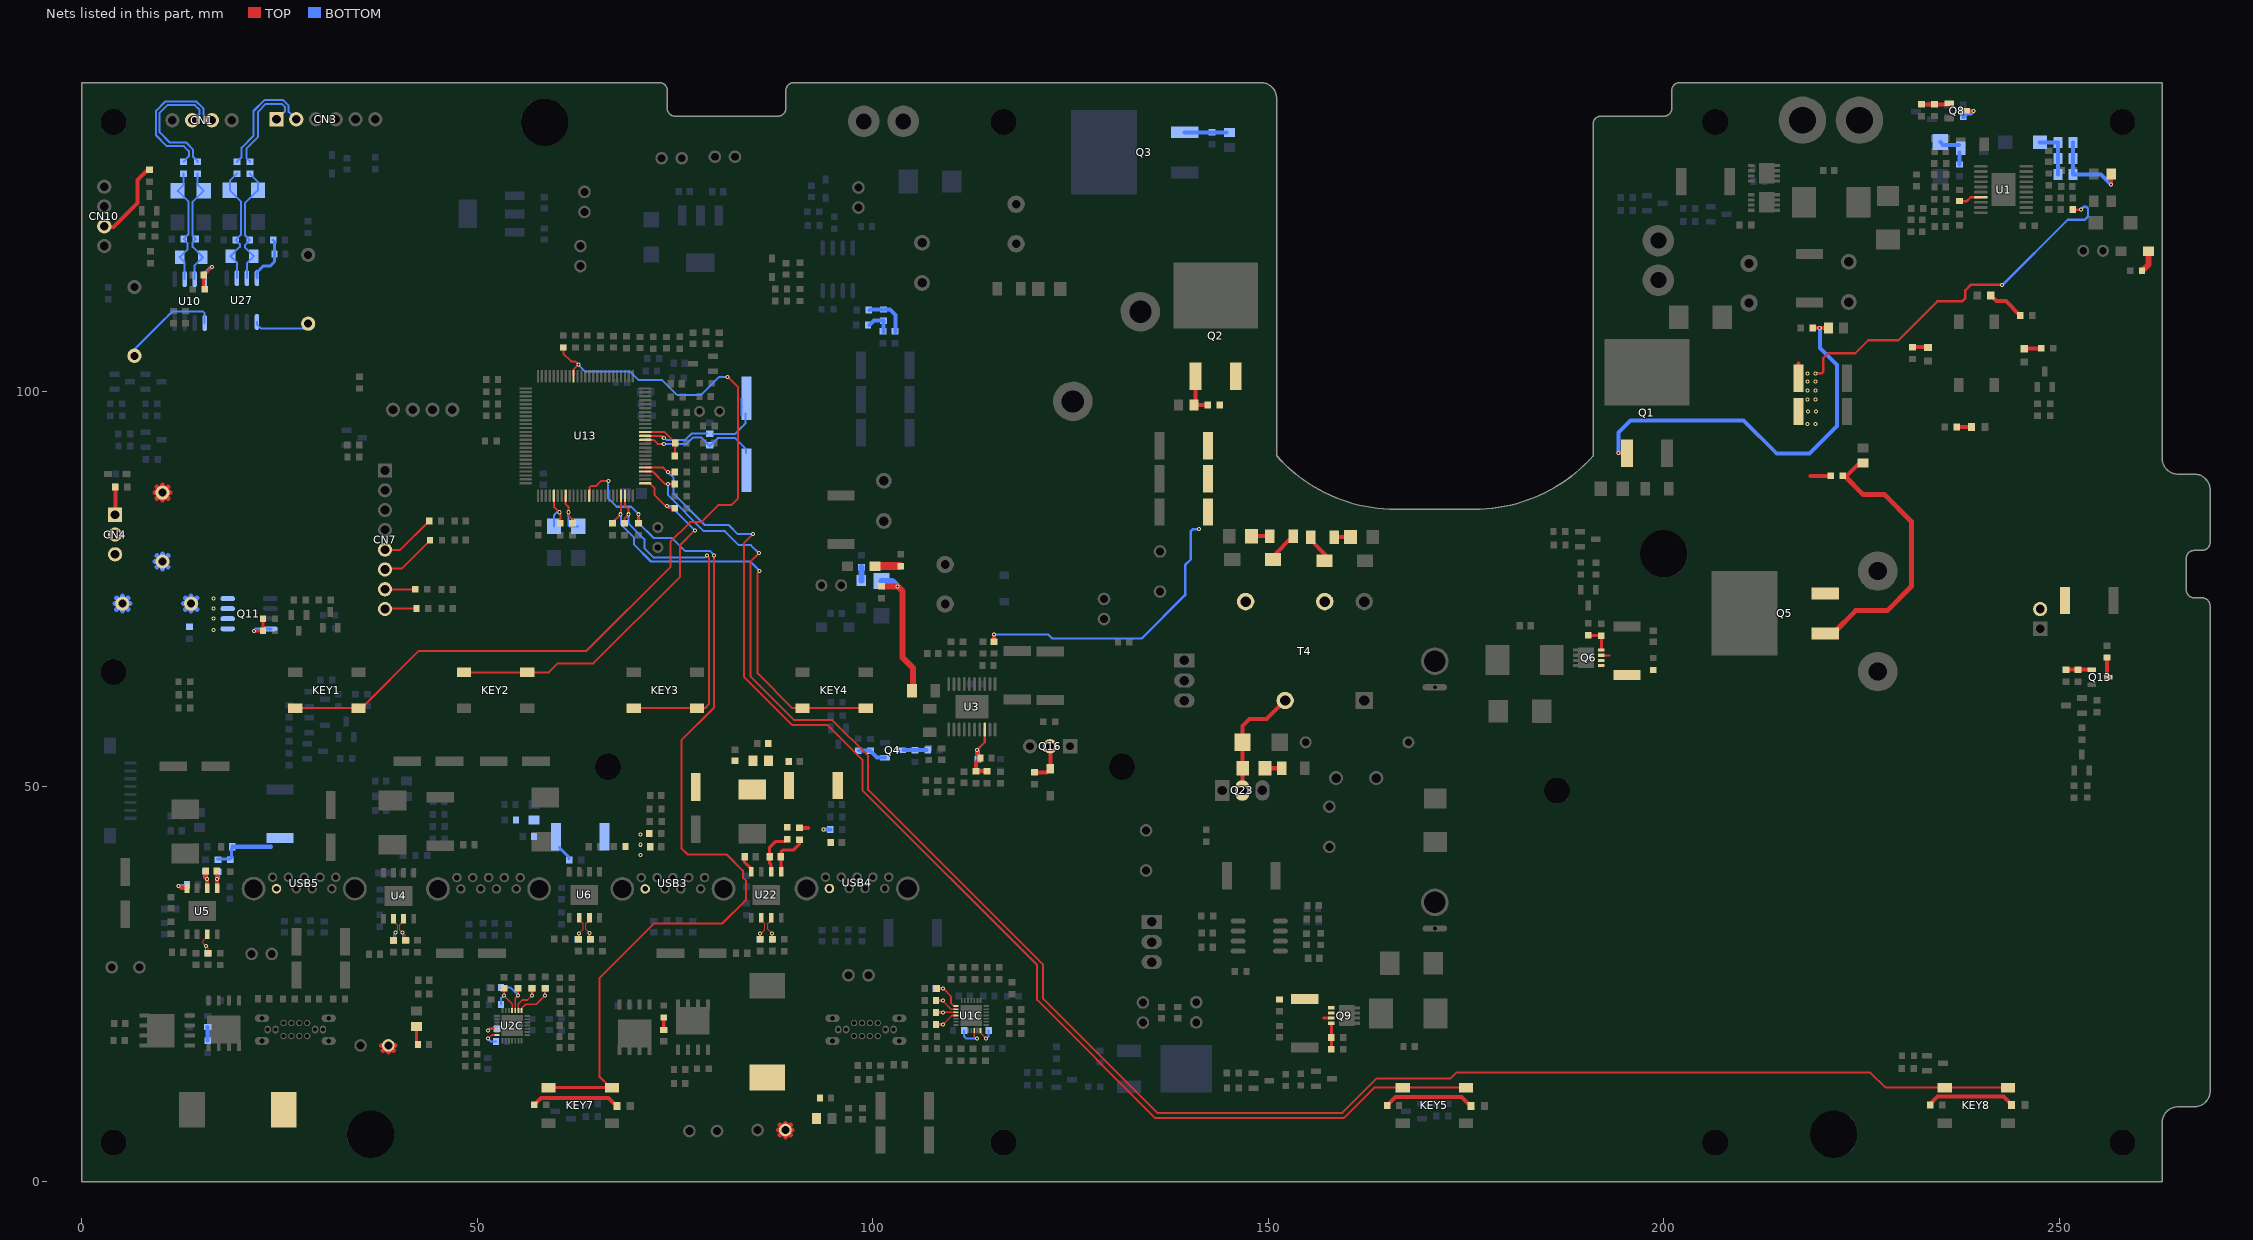
[diagram p0: the nets of this part, all layers, seen from the top]
# Altium PCB MISC84402.PcbDoc (part 7 of 12)
Units mm, origin at the board's own origin, x right, y up, seen from the top; angles counter-clockwise.
Board outline 269.06 x 139 mm, 4 copper layers (TOP, GND02, PWR03, BOTTOM), stack 0.732 mm thick; 694 components, 428 nets, 1859 pads, 1384 vias.

## Via types
v1: diameter 0.508, hole 0.254, TOP to BOTTOM, tented both sides, 1015 vias
v2: diameter 0.508, hole 0.254, TOP to BOTTOM, 243 vias
v3: diameter 0.508, hole 0.305, TOP to BOTTOM, 60 vias
v4: diameter 0.61, hole 0.305, TOP to BOTTOM, 55 vias
v5: diameter 0.61, hole 0.305, TOP to BOTTOM, tented both sides, 8 vias
v6: diameter 0.762, hole 0.381, TOP to BOTTOM, 2 vias
v7: diameter 0.762, hole 0.381, TOP to BOTTOM, tented both sides, 1 vias

## Nets (pads, with @x,y where several pads share a name; then routed paths per layer and width w, separated by ;. In a path a pad name is that pad's centre, name@x,y a point inside that pad or via, vN(x,y) a via of type N, cw(c..) or ccw(c..) an arc to the next point about the centre after c; other vN are vias at no path point) (continued)
NETC107_1: C107.1 C113.2 L6.2 L13.1 | length 7.1
  TOP w0.635: 88.075,6.569 C107.1@88.926,6.569 ; 88.273,5.916 C107.1@88.926,6.569 ; 88.273,7.221 C107.1@88.926,6.569 ; 88.926,5.717 C107.1@88.926,6.569 ; 88.926,7.42 C107.1@88.926,6.569 ; 89.579,5.916 C107.1@88.926,6.569 ; 89.579,7.221 C107.1@88.926,6.569 ; 89.777,6.569 C107.1@88.926,6.569
NETC108_1: C108.1 R166.2 U1C.3 | length 3.4
  TOP w0.203: C108.1@108.179,21.463 108.195,21.447 U1C.3@110.513,21.447
  TOP w0.254: C108.1@107.978,21.428 C108.1@108.179,21.428
  BOTTOM w0.254: R166.2@107.978,21.428 v1(108.865,21.428)
NETC109_1: C109.1 R204.2 U2C.3 | length 5.5
  TOP w0.203: U2C.3@54.782,21.684 54.782,23.225 v1(55.144,23.587)
  TOP w0.254: v1(55.144,23.587) C109.1@55.144,24.476
  BOTTOM w0.254: R204.2@52.976,24.603 54.128,24.603 v1(55.144,23.587)
NETC110_1: C110.1 R160.2 U1C.1 | length 4.8
  TOP w0.203: R160.2@108.28,24.486 108.89,24.486 109.88,23.495 109.88,22.581 110.214,22.247 U1C.1@110.513,22.247
  TOP w0.254: R160.2@108.083,24.476 R160.2@108.28,24.476
  BOTTOM w0.254: C110.1@107.976,24.476 v1(108.867,24.476)
NETC111_1: C111.1 R205.2 U2C.2 | length 4.8
  TOP w0.203: U2C.2@55.182,21.684 55.182,22.543 55.651,23.012 56.337,23.012 56.972,23.647 C111.1@56.972,24.333
  TOP w0.254: C111.1@56.922,24.333 C111.1@56.922,24.476
  BOTTOM w0.254: v1(56.922,23.587) R205.2@56.922,24.476
NETC115_1: C115.1 C129.2 L7.2 L12.1 | length 6.8
  TOP w0.381: L12.1@42.291,19.685 42.291,17.588 C129.2@42.48,17.399
  TOP w0.635: 37.882,17.265 C115.1@38.733,17.265 ; 38.08,16.612 C115.1@38.733,17.265 ; 38.733,16.413 C115.1@38.733,17.265 ; 39.386,16.612 C115.1@38.733,17.265 ; 39.584,17.265 C115.1@38.733,17.265
NetC117_2: C117.2 C142.2 L11.2 R82.2 R340.1 | length 1.9
  BOTTOM w0.381: R82.2@60.376,42.266 61.578,41.063 R340.1@61.578,40.853
NETC118_1: C118.1 R229.1 U10.8 | length 5.3
  TOP w0.381: R229.1@15.52,112.868 15.395,112.992 C118.1@15.395,114.646 v1(16.431,115.681)
  BOTTOM w0.381: U10.8@15.52,114.138 15.52,114.9 16.301,115.681 v1(16.431,115.681)
NETC119_2: C119.2 R174.1 | length 1.6
  TOP w0.381: C119.2@73.559,19.207 R174.1@73.559,20.801
NETC120_2: C120.2 U1C.14 | length 2.5
  TOP w0.203: U1C.14@113.621,19.139 113.621,18.84 v1@114.3,18.161
  TOP w0.254: v1@114.295,18.156 v1(114.326,18.126)
  BOTTOM w0.254: v1(114.326,18.126) 114.645,18.444 C120.2@114.645,19.142
NETC121_2: C121.2 U2C.12 | length 2.5
  TOP w0.203: v1@51.333,19.101 51.609,19.377 U2C.12@52.474,19.377
  BOTTOM w0.254: v1(51.334,19.142) 51.569,19.377 C121.2@52.474,19.377
NetC123_2: C123.2 C150.2 L14.2 R83.2 R339.1
NETC124_1: C124.1 R231.1 U27.8 | length 6.3
  BOTTOM w0.381: U27.8@22.124,114.265 22.124,115.027 22.886,115.789 23.775,115.789 24.345,116.359 C124.1@24.345,117.313 24.345,118.91 R231.1@24.165,119.091
NetC130_2: C130.2 R7.2 R8.1 R14.1 U3.8 | length 8.7
  TOP w0.305: v1(113.157,54.61) 114.147,55.6 U3.8@114.147,57.198
  TOP w0.508: v1(113.157,54.61) 113.157,54.037 C130.2@113.6,53.594 113.03,53.024 R14.1@113.03,51.934 R8.1@114.427,51.934
  BOTTOM w0.508: v1(113.157,54.61) 113.284,54.483 R7.2@113.284,53.467
NETC132_1: C132.1 R203.2 U2C.1 | length 5.7
  TOP w0.203: U2C.1@55.582,21.684 55.582,21.952 56.109,22.479 57.455,22.479 58.572,23.597 R203.2@58.572,24.359
  TOP w0.254: R203.2@58.573,24.359 R203.2@58.573,24.476
  BOTTOM w0.254: v1(58.573,23.587) C132.1@58.573,24.476
NETC134_1: C134.1 R208.2 U2C.4 | length 4.5
  TOP w0.203: C134.1@53.391,24.409 53.391,23.562 53.391,23.52 54.382,22.529 U2C.4@54.382,21.684
  TOP w0.254: C134.1@53.366,24.409 C134.1@53.366,24.476
  BOTTOM w0.254: R208.2@52.976,22.444 52.976,23.197 v1(53.366,23.587)
NETC135_1: C135.1 R164.2 U1C.2 | length 3.9
  TOP w0.203: C135.1@108.026,22.936 108.788,22.936 109.878,21.847 U1C.2@110.513,21.847
  TOP w0.254: C135.1@107.978,22.952 C135.1@108.026,22.952
  BOTTOM w0.254: R164.2@107.978,22.952 v1(108.865,22.952)
NETC136_2: C136.2 U2C.14 | length 2.5
  TOP w0.203: v1@51.384,18.161 51.8,18.577 U2C.14@52.474,18.577
  TOP w0.254: v1(51.334,18.126) v1@51.377,18.168
  BOTTOM w0.254: v1(51.334,18.126) 51.715,17.745 C136.2@52.35,17.745
NETC139_2: C139.2 R226.1 | length 1.7
  BOTTOM w0.508: R226.1@15.901,17.863 C139.2@15.901,19.585
NETC143_1: C143.1 R344.2 U5.1 | length 3.3
  TOP w0.508: C143.1@17.046,39.335 v1(17.046,38.319) 17.098,38.267 U5.1@17.098,37.163
  BOTTOM w0.508: v1(17.046,38.319) 17.171,38.443 R344.2@17.171,39.335
NETC143_2: C143.2 R345.2 U5.2 | length 3.4
  TOP w0.508: C143.2@15.647,39.335 15.647,38.503 v1(15.828,38.322) U5.2@15.828,37.163
  BOTTOM w0.508: R345.2@15.647,39.352 15.647,38.503 v1(15.828,38.322)
NETC145_2: C145.2 U5.4 | length 2.3
  TOP w0.508: v1(12.218,37.43) 12.345,37.43 12.612,37.163 U5.4@13.288,37.163
  BOTTOM w0.508: v1(12.218,37.43) 13.28,37.43 C145.2@13.296,37.43
NETC146_1: C146.1 R167.2 U1C.4 | length 3.9
  TOP w0.203: v1(108.865,19.904) 110.008,21.047 U1C.4@110.513,21.047
  TOP w0.254: C146.1@107.978,19.904 v1(108.865,19.904)
  BOTTOM w0.254: R167.2@107.978,19.904 v1(108.865,19.904)
NETC148_1: C148.1 R241.2 U22.1 | length 5.9
  TOP w0.381: U22.1@88.418,39.195 88.418,39.969 88.356,40.032 C148.1@88.356,41.113 88.356,41.685 88.672,42.002 90.008,42.002 90.704,42.698 R241.2@90.704,43.281
NETC148_2: C148.2 R339.2 U22.2 | length 5.8
  TOP w0.381: U22.2@87.148,39.195 87.148,40.097 86.956,40.289 C148.2@86.956,41.113 86.956,42.318 87.656,43.018 88.917,43.018 R339.2@89.18,43.281
NETC149_2: C149.2 U13.13 X1.1 | length 16.4
  TOP w0.254: U13.13@71.203,94.326 73.305,94.326 v1(73.559,94.072)
  BOTTOM w0.254: v1@73.635,94.082 73.889,93.828 76.276,93.828 77.064,94.615 C149.2@79.045,94.615 ; C149.2@79.784,94.539 82.525,94.539 83.312,95.326 83.414,95.428 83.896,95.91 X1.1@83.896,97.155 ; X1.1@83.414,96.926 X1.1@83.414,97.892 ; X1.1@83.414,99.073 X1.1@83.414,97.892 ; X1.1@83.439,97.917 X1.1@83.414,97.892
NETC151_2: C151.2 U22.4 | length 2.3
  TOP w0.381: C151.2@83.781,41.113 83.781,40.416 84.608,39.589 U22.4@84.608,39.195
NetC153_2: C153.2 C160.1 L10.2 L14.1
NetC154_2: C154.2 R359.2 | length 2.1
  TOP w0.508: C154.2@147.873,81.652 R359.2@149.996,81.652
NETC155_1: C155.1 R112.1 R268.2 | length 3.5
  BOTTOM w0.508: R112.1@99.552,108.331 100.122,108.901 C155.1@101.346,108.901 R268.2@101.346,107.433
NETC155_2: C155.2 R281.2 R290.1 | length 5.8
  BOTTOM w0.508: R290.1@99.552,110.236 99.617,110.301 C155.2@101.346,110.301 102.17,110.301 102.87,109.601 R281.2@102.87,107.433
NetC157_2: C157.2 R360.2 | length 1.7
  TOP w0.508: R360.2@158.315,81.525 C157.2@160.004,81.525
NetC158_1: C158.1 R361.2 | length 2.2
  TOP w0.381: C158.1@149.567,52.308 C158.1@149.8,52.308 ; R361.2@151.444,52.308 R361.2@151.536,52.4
  TOP w0.508: C158.1@149.8,52.308 R361.2@151.666,52.308
NetC158_2: C158.2 D20.2 Q23.2 T4.3 | length 14.9
  TOP w0.508: Q23.2@146.711,49.495 D20.2@146.711,55.591 146.711,57.623 147.6,58.512 149.766,58.512 T4.3@152.125,60.871
NETC163_2: C163.2 U13.12 X1.2 | length 15
  TOP w0.254: U13.12@71.203,93.826 72.281,93.826 72.797,93.31 v1(73.559,93.31)
  BOTTOM w0.254: 73.823,93.32 76.479,93.32 77.299,94.139 78.302,94.139 79.388,93.053 80.366,94.031 82.601,94.031 83.947,92.685 X1.2@83.947,92.151
NETC164_2: C164.2 R293.1 U13.14 | length 6.1
  TOP w0.254: U13.14@71.203,94.826 73.629,94.826 C164.2@75.018,93.437 75.018,92.802 74.965,92.748 R293.1@74.965,91.786
NetC165_2: C165.2 R242.2 U5.7 | length 3.3
  TOP w0.127: U5.7@15.828,31.346 15.828,31.006 15.364,30.543 15.364,30.124 15.658,29.831 v2(15.672,29.817) 15.951,29.537 R242.2@15.951,29.159
  BOTTOM w0.127: C165.2@15.646,29.159 15.672,29.185 v2(15.672,29.817)
NetC166_2: C166.2 R89.2 U4.6 | length 3.8
  TOP w0.127: U4.6@39.396,33.251 39.396,32.984 39.929,32.452 39.929,31.801 v2@39.624,31.496 ; R89.2@39.421,30.785 39.421,31.293 v2@39.624,31.496 ; v2(39.624,31.521) v2@39.624,31.496
  BOTTOM w0.127: C166.2@39.599,30.683 39.624,30.709 v2(39.624,31.521)
NetC169_2: C169.2 R81.2 U4.7 | length 3.9
  TOP w0.127: v2(40.526,31.559) v2@40.5,31.559 ; U4.7@40.666,33.251 40.666,32.984 40.202,32.521 40.202,31.857 v2@40.5,31.559 ; R81.2@40.838,30.653 R81.2@40.92,30.572 ; R81.2@40.894,30.709 40.894,31.166 v2@40.5,31.559
  BOTTOM w0.127: v2(40.526,31.559) 40.615,31.471 C169.2@40.615,30.81
NETC170_2: C170.2 R82.1 R87.1 R341.1 USB3.1
  other v1: 70.638,41.367 70.638,42.637 70.638,43.907
NetC173_2: C173.2 R111.2 U6.6 | length 3.4
  TOP w0.127: R111.2@62.789,30.963 v2@62.789,31.369 ; v2(62.814,31.445) 62.84,31.42 63.354,31.935 63.354,32.648 62.891,33.112 U6.6@62.891,33.378
  BOTTOM w0.127: C173.2@62.789,30.886 62.814,30.912 v2(62.814,31.445)
NetC174_2: C174.2 R238.2 U6.7 | length 3.4
  TOP w0.127: v2(64.16,31.471) 64.135,31.496 63.697,31.934 63.697,32.648 64.161,33.112 U6.7@64.161,33.378 ; R238.2@64.237,30.937 v2@64.237,31.394
  BOTTOM w0.127: C174.2@64.135,30.861 64.16,30.886 v2(64.16,31.471)
NetC175_2: C175.2 R247.2 U22.6 | length 3.5
  TOP w0.127: R247.2@85.75,30.861 v2@85.75,31.267 ; v2(85.75,31.394) 85.814,31.331 86.341,31.858 86.341,32.648 85.878,33.112 U22.6@85.878,33.378
  BOTTOM w0.127: v2(85.75,31.394) 85.75,30.861 C175.2@85.776,30.836
NetC177_2: C177.2 R245.2 U22.7 | length 3.9
  TOP w0.127: U22.7@87.148,33.378 87.148,33.112 86.684,32.648 86.684,31.934 v2@87.249,31.369 ; R245.2@87.206,30.767 R245.2@87.275,30.699 ; R245.2@87.249,30.81 v2@87.249,31.369 ; v2(87.249,31.445) v2@87.249,31.369
  BOTTOM w0.127: C177.2@87.249,30.759 v2(87.249,31.445)
NETC179_2: C179.2 U1C.12 | length 3.7
  TOP w0.203: U1C.12@112.821,19.139 112.821,18.361 113.042,18.139 v1(113.183,18.139)
  BOTTOM w0.254: C179.2@111.534,19.142 111.534,18.393 111.788,18.139 v1(113.183,18.139)
NETC192_2: C192.2 R31.1 R63.1 R344.1 USB5.1 | length 7.8
  BOTTOM w0.381: R344.1@17.171,40.841 18.743,40.841 18.898,40.996 C192.2@18.898,42.088
  BOTTOM w0.508: C192.2@19.014,42.383 23.902,42.383
NETC194_1: C194.1 U1.7 | length 2.9
  TOP w0.305: C194.1@237.363,124.014 238.314,124.014 238.801,124.501 U1.7@240.078,124.501
NETC199_2: C199.2 R83.1 R96.1 R241.1 USB4.1 | length 2
  TOP w0.508: R241.1@90.703,44.781 91.797,44.781
  BOTTOM w0.508: v1(93.726,44.577) 94.598,44.577 R96.1@94.615,44.577 ; R96.1@94.624,44.577 R96.1@94.615,44.577 ; R96.1@94.64,44.552 R96.1@94.615,44.577
NETCN1_2: CN1.2 R225.2 | length 16.4
  BOTTOM w0.254: CN1.2@14.326,134.442 14.859,134.976 14.859,135.56 14.275,136.144 10.795,136.144 9.83,135.179 9.83,132.69 11.1,131.42 13.183,131.42 14.072,130.531 14.072,129.591 14.631,129.032 R225.2@14.631,128.979
NetCN1_3: CN1.3 R234.2 | length 18.1
  BOTTOM w0.254: R234.2@12.853,128.997 13.513,129.657 13.513,130.327 12.878,130.962 10.719,130.962 9.373,132.309 9.373,135.458 10.516,136.601 14.453,136.601 15.392,135.661 15.392,134.899 CN1.3@15.951,134.341
NETCN3_1: CN3.1 R233.2 | length 12.1
  BOTTOM w0.254: R233.2@21.235,128.979 21.235,129.057 20.777,129.515 20.777,130.632 22.276,132.131 22.276,135.306 23.266,136.296 25.273,136.296 25.679,135.89 25.679,135.407 CN3.1@25.298,135.026
NETCN3_2: CN3.2 R235.2 | length 14.5
  BOTTOM w0.254: R235.2@19.584,128.979 20.193,129.588 20.193,130.759 21.692,132.258 21.692,135.407 23.063,136.779 25.425,136.779 26.137,136.068 26.137,135.306 CN3.2@26.924,134.518
NETCN4_1: CN4.1 R298.1 | length 2.9
  TOP w0.508: CN4.1@4.217,84.938 R298.1@4.217,87.849
NETCN4_2: CN4.2 D10.2 Q11.5 Q11.6 Q11.7 Q11.8 | length 7.9
  TOP w0.635: 9.234,87.151 D10.2@10.186,87.151 ; 9.462,86.427 D10.2@10.186,87.151 ; 9.462,87.874 D10.2@10.186,87.151 ; 10.186,86.199 D10.2@10.186,87.151 ; 10.186,88.102 D10.2@10.186,87.151 ; 10.91,86.427 D10.2@10.186,87.151 ; 10.91,87.874 D10.2@10.186,87.151 ; 11.137,87.151 D10.2@10.186,87.151
  other v1: 16.663,69.815 16.663,71.212 16.663,72.482 16.663,73.752
NETCN4_3: CN4.3 D5.1 D10.1 | length 14.8
  BOTTOM w0.635: 4.154,73.117 D5.1@5.106,73.117 ; 4.382,72.393 D5.1@5.106,73.117 ; 4.382,73.84 D5.1@5.106,73.117 ; 5.106,72.165 D5.1@5.106,73.117 ; 5.106,74.068 D5.1@5.106,73.117 ; 5.83,72.393 D5.1@5.106,73.117 ; 5.83,73.84 D5.1@5.106,73.117 ; 6.057,73.117 D5.1@5.106,73.117 ; 9.234,78.451 D10.1@10.186,78.451 ; 9.462,77.727 D10.1@10.186,78.451 ; 9.462,79.174 D10.1@10.186,78.451 ; 10.186,77.499 D10.1@10.186,78.451 ; 10.186,79.402 D10.1@10.186,78.451 ; 10.91,77.727 D10.1@10.186,78.451 ; 10.91,79.174 D10.1@10.186,78.451
NetCN7_5: CN7.5 R207.2 | length 6.7
  TOP w0.254: CN7.5@38.684,79.908 40.227,79.908 R207.2@43.888,83.569
NetCN7_6: CN7.6 R254.2 | length 6.8
  TOP w0.254: CN7.6@38.659,77.546 40.429,77.546 R254.2@44.01,81.128
NetCN7_7: CN7.7 R255.2 | length 3.6
  TOP w0.254: CN7.7@38.557,74.93 R255.2@42.164,74.93
NetCN7_8: CN7.8 R264.2 | length 3.4
  TOP w0.254: CN7.8@38.862,72.517 R264.2@42.291,72.517
NetCN10_2: CN10.2 R363.1 | length 10.3
  TOP w0.508: CN10.2@2.896,120.752 3.962,120.752 7.01,123.8 7.01,126.695 8.28,127.965 R363.1@8.551,127.965
NETCON1_2: CON1.2 R368.2
NETD2_1: D2.1 R6.2 R330.1 | length 4
  BOTTOM w0.508: D2.1@234.95,131.486 235.321,131.115 R330.1@237.287,131.115 ; R6.2@237.363,128.642 R330.1@237.363,130.184
NETD3_1: D3.1 R9.2 R331.1 | length 18.4
  TOP w0.762: R9.2@101.092,75.302 v1(103.133,75.302) 103.768,74.667 103.768,66.285 105.08,64.973 R331.1@105.08,62.103
  BOTTOM w0.762: D3.1@101.092,75.996 102.439,75.996 v1(103.133,75.302)
NetD4_2: D4.2 R362.2 | length 3.1
  TOP w1.016: D4.2@100.278,77.876 R362.2@103.403,77.876
NETD5_2: D5.2 R197.2 | length 6.9
  BOTTOM w0.635: 12.854,73.117 D5.2@13.806,73.117 ; 13.082,72.393 D5.2@13.806,73.117 ; 13.082,73.84 D5.2@13.806,73.117 ; 13.806,72.165 D5.2@13.806,73.117 ; 13.806,74.068 D5.2@13.806,73.117 ; 14.53,72.393 D5.2@13.806,73.117 ; 14.53,73.84 D5.2@13.806,73.117
NetD13_2: D13.2 R360.1 T4.7 | length 3.1
  TOP w0.508: R360.1@155.358,81.525 155.358,81.167 D13.2@157.302,79.223
NetD15_2: D15.2 R48.1 | length 2.7
  TOP w0.762: R48.1@260.604,115.316 261.289,116.001 D15.2@261.289,117.694
NETD23_2: D23.2 R327.1 R328.1 R329.1 | length 10.7
  TOP w0.508: v1(256.54,126.111) D23.2@256.54,127.465
  BOTTOM w0.508: R328.1@251.757,131.445 R329.1@251.757,129.413 R327.1@251.757,127.381 255.27,127.381 v1(256.54,126.111)
NETD26_1: D26.1 U10.1 | length 13
  BOTTOM w0.254: D26.1@6.63,104.454 6.63,105.248 10.567,109.185 10.576,109.185 10.948,109.557 10.948,109.566 11.456,110.074 15.266,110.074 15.52,109.82 U10.1@15.52,108.603
NETD27_1: D27.1 U27.1 | length 7.2
  BOTTOM w0.254: U27.1@22.124,108.73 22.124,108.423 22.632,107.915 27.998,107.915 D27.1@28.601,108.518
NETD39_2: D39.2 R326.1 | length 1.7
  BOTTOM w0.762: D39.2@98.552,76.03 R326.1@98.552,77.733
NETD42_1: D42.1 R220.1 R232.2 R234.1 U10.6 | length 15.4
  BOTTOM w0.254: R234.1@12.853,127.49 12.853,126.076 D42.1@12.091,125.314 13.488,123.917 13.488,119.853 12.853,119.218 13.361,118.709 13.361,117.948 R220.1@12.345,116.932 12.98,116.297 U10.6@12.98,114.138
NETD43_1: D43.1 R192.1 R220.2 R225.1 U10.7 | length 15.5
  BOTTOM w0.254: U10.7@14.25,114.138 14.25,115.879 R220.2@15.302,116.932 13.996,118.238 13.996,118.819 14.394,119.218 13.996,119.616 13.996,123.917 D43.1@15.393,125.314 14.631,126.076 R225.1@14.631,127.473
NETD44_1: D44.1 R230.1 R233.1 R239.1 U27.7 | length 15.7
  BOTTOM w0.254: U27.7@20.854,114.265 20.854,116.17 R239.1@21.743,117.059 20.6,118.202 20.6,118.456 R230.1@21.235,119.091 20.6,119.726 20.6,123.726 D44.1@22.251,125.377 22.251,126.457 R233.1@21.235,127.473
NETD45_1: D45.1 R235.1 R239.2 R244.2 U27.6 | length 15.5
  BOTTOM w0.254: U27.6@19.584,114.265 19.584,116.26 R239.2@18.785,117.059 19.965,118.238 19.965,118.565 R244.2@19.439,119.091 20.092,119.743 20.092,123.98 D45.1@18.695,125.377 18.695,126.584 R235.1@19.584,127.473
NETD46_2: D46.2 R324.2 U13.80 | length 5.9
  TOP w0.254: U13.80@59.653,86.776 59.653,85.372 v1(60.351,84.674) ; R324.2@60.478,83.268 v1@60.478,84.547
  BOTTOM w0.254: D46.2@59.69,82.899 59.69,84.328 60.036,84.674 v1(60.351,84.674)
NETD47_2: D47.2 R47.2 U13.83 | length 6.8
  TOP w0.254: U13.83@61.153,86.776 61.153,85.71 61.494,85.369 v1(61.494,84.674) 61.494,84.293 62.002,83.785 R47.2@62.002,83.277
  BOTTOM w0.254: v1(61.494,84.674) 61.494,83.032 61.627,82.899 D47.2@62.738,82.899
NETD48_1: D48.1 Q16.2 R20.2 | length 4.4
  TOP w0.508: R20.2@120.447,51.797 121.977,51.797 122.428,52.248 Q16.2@122.428,54.432
NETD50_2: D50.2 R327.2 R328.2 R329.2 | length 6.3
  BOTTOM w0.508: D50.2@247.556,131.445 R328.2@249.825,131.445 R329.2@249.825,129.413 R327.2@249.825,127.381
NETD62_2: D62.2 R359.1 T4.5 | length 3.2
  TOP w0.508: D62.2@150.774,79.197 150.774,79.294 R359.1@152.998,81.518
NETKEY1_3: KEY1.3 KEY1.4 R3.2 U13.41 | length 111.1
  TOP w0.254: KEY1.3@26.964,59.919 35.343,59.92 42.571,67.148 63.788,67.148 74.384,77.744 74.384,80.927 76.764,83.307 ; R3.2@60.859,105.51 60.859,104.74 61.84,103.759 62.348,103.759 v1(62.764,103.343) 62.153,102.732 U13.41@62.153,101.876 ; 76.759,83.312 76.86,83.414 78.283,83.414 80.432,85.563 82.068,85.563 82.957,86.452 82.957,100.482 v2(81.636,101.803) v2@81.61,101.803
  BOTTOM w0.254: v1(62.764,103.343) 63.653,102.454 69.301,102.454 70.383,101.371 73.355,101.371 75.209,99.517 78.308,99.517 80.594,101.803 v2@81.61,101.803
NETKEY2_1: KEY2.1 KEY2.2 R252.1 U13.1 | length 49.5
  TOP w0.254: KEY2.1@48.3,64.419 KEY2.2@56.3,64.419 59.019,64.419 60.158,65.557 64.668,65.557 75.591,76.48 75.591,80.474 v1(77.5,82.383) ; U13.1@71.203,88.326 71.781,88.326 72.416,87.691 72.416,86.833 73.813,85.436 v1(73.94,85.436) 74.194,85.182 R252.1@74.956,85.182
  BOTTOM w0.254: v1@73.94,85.308 v1(73.94,85.436) 74.448,85.436 v1(77.5,82.383)
NETKEY3_3: KEY3.3 KEY3.4 R251.1 U13.98 | length 46.1
  TOP w0.254: R251.1@68.606,83.277 68.606,83.912 v1(69.114,84.42) 69.114,85.055 68.653,85.516 U13.98@68.653,86.776 ; KEY3.3@69.763,59.919 KEY3.4@77.763,59.919 78.777,59.92 79.274,60.417 79.274,78.959 v1(79.02,79.213)
  BOTTOM w0.254: v1@69.063,84.379 v1@69.113,84.328 ; v1@69.088,84.303 69.088,83.287 71.095,81.28 71.095,80.137 72.288,78.943 78.75,78.943 v1(79.02,79.213)
NETKEY4_3: KEY4.3 KEY4.4 R250.1 U13.97 | length 54.3
  TOP w0.254: R250.1@67.082,83.277 67.082,83.404 v1(68.098,84.42) 68.153,84.475 U13.97@68.153,86.776 ; v1(85.687,77.244) 85.42,76.977 85.42,64.303 89.804,59.92 KEY4.4@99.099,59.919
  BOTTOM w0.254: v1(68.098,84.42) v1@68.131,84.387 ; v1@68.123,84.379 68.123,83.16 69.774,81.509 69.774,80.62 71.943,78.451 84.481,78.451 v1(85.687,77.244)
NetKEY5_1: KEY5.1 KEY5.2 R221.1 U13.5 | length 158.6
  TOP w0.254: U13.5@71.203,90.326 73.495,90.326 v1(74.067,89.754) R221.1@74.956,89.754 ; v1(84.836,81.915) 83.693,80.772 83.693,63.872 89.805,57.76 94.285,57.76 98.679,53.365 98.679,49.53 120.777,27.432 120.777,23.012 135.712,8.077 159.537,8.077 163.379,11.919 KEY5.2@175,11.919
  BOTTOM w0.254: v1(74.067,89.754) 74.803,89.018 74.803,86.995 78.74,83.058 81.788,83.058 82.931,81.915 v1(84.836,81.915)
NetKEY7_1: KEY7.1 KEY7.2 R228.1 U13.89 | length 120.2
  TOP w0.254: U13.89@64.153,86.776 64.153,87.791 64.373,88.011 65.024,88.011 65.659,88.646 v1(66.548,88.646) ; KEY7.2@66.65,12.09 65.405,13.335 65.405,25.756 72.314,32.664 80.924,32.664 83.963,35.703 83.963,38.084 83.566,38.481 83.566,39.37 81.534,41.402 76.581,41.402 75.776,42.207 75.776,55.837 79.909,59.97 v1(79.909,79.222) ; R228.1@70.384,83.277 v1(70.384,84.42)
  TOP w0.381: KEY7.1@59,11.919 KEY7.2@66.65,11.919
  BOTTOM w0.254: v1@66.523,88.671 66.523,86.436 67.589,85.369 69.434,85.369 v1(70.384,84.42) v1@70.442,84.361 ; v1@70.358,84.303 70.358,83.337 72.263,81.432 74.574,81.432 76.225,79.781 79.4,79.781 v1@79.832,79.35 ; v1(79.909,79.222) v1@79.909,79.35
NETKEY8_1: KEY8.1 KEY8.2 R219.1 U13.4 | length 226.1
  TOP w0.254: U13.4@71.203,89.826 72.174,89.826 73.769,88.23 v1(74.067,88.23) R219.1@74.956,88.23 ; v1(85.598,79.502) 84.557,78.461 84.557,63.897 90.059,58.395 94.869,58.395 99.39,53.873 99.39,49.581 121.514,27.457 121.514,23.19 135.966,8.738 159.36,8.738 163.728,13.106 173.05,13.106 173.778,13.835 226.119,13.835 228.034,11.92 KEY8.2@243.5,11.92
  BOTTOM w0.254: v1(74.067,88.23) 74.067,86.867 78.638,82.296 81.28,82.296 83.058,80.518 84.582,80.518 v1(85.598,79.502)
NETLED1_2: LED1.2 R64.1 | length 10.6
  TOP w0.508: R64.1@233.756,9.982 234.594,10.82 242.951,10.82 LED1.2@243.713,10.058
NETLED2_2: LED2.2 R78.1 | length 2.2
  TOP w0.508: LED2.2@245.618,105.385 245.643,105.359 R78.1@247.786,105.359
NETLED3_2: LED3.2 R194.1 | length 10.8
  TOP w0.508: R194.1@57.184,9.754 58.048,10.617 66.573,10.617 LED3.2@67.31,9.881
NetLED4_2: LED4.2 R195.1 | length 11.3
  TOP w0.508: R195.1@165.007,9.652 166.099,10.744 174.396,10.744 LED4.2@175.438,9.703
NetLED5_2: LED5.2 R79.1 | length 1.9
  TOP w0.508: R79.1@231.445,105.554 LED5.2@233.359,105.554
NetLED6_2: LED6.2 R118.1 | length 1.6
  TOP w0.508: R118.1@237.321,95.437 LED6.2@238.884,95.437
NetLED7_2: LED7.2 R187.1 | length 4.7
  TOP w0.508: LED7.2@241.329,112.081 242.056,111.354 243.256,111.354 R187.1@245.034,109.576
NETQ1_1: Q1.1 R121.1 R253.2 | length 51.1
  TOP w0.508: v1(194.259,92.151) Q1.1@195.021,92.151 ; Q1.1@195.326,91.059 Q1.1@195.326,92.149 ; R253.2@218.812,107.95 v1(219.71,107.95) R121.1@220.81,107.95
  BOTTOM w0.508: v1@194.285,92.177 194.285,94.767 195.783,96.266 210.083,96.266 214.274,92.075 218.389,92.075 221.869,95.555 221.869,103.302 219.735,105.435 219.735,107.925 v1(219.71,107.95)
NETQ2_1: Q2.1 R101.1 R261.2 | length 6.5
  TOP w0.508: Q2.1@140.565,101.853 Q2.1@140.565,102.997 ; R101.1@140.582,98.273 R101.1@140.582,98.222 R261.2@142.325,98.222 ; R101.1@140.792,98.273 Q2.1@140.792,101.853
NetQ2_3: Q2.3 R4.2 R5.2 R25.1 R41.2 R261.1 | length 37.1
  TOP w0.508: R25.1@115.316,68.317 v1(115.316,69.215)
  BOTTOM w0.305: v1(115.316,69.215) 122.174,69.215 122.682,68.707 133.985,68.707 139.471,74.193 139.471,78.003 140.208,78.74 140.208,82.296 140.462,82.55 v1(141.224,82.55)
NETQ3_1: Q3.1 R74.1 R260.2 | length 5.3
  BOTTOM w0.508: Q3.1@139.422,132.715 139.431,132.706 R260.2@142.875,132.706 R74.1@144.687,132.706
NetQ4_1: Q4.1 R104.2 R291.2 | length 3.6
  BOTTOM w0.508: R104.2@98.273,54.559 99.644,54.559 100.543,53.66 Q4.1@101.54,53.66
NetQ4_3: Q4.3 R37.1 R51.2 | length 2.9
  BOTTOM w0.508: Q4.3@103.844,54.601 R51.2@105.308,54.601 R37.1@106.747,54.601
NETQ5_1: Q5.1 R125.1 R259.2 | length 34.4
  TOP w0.381: R125.1@225.162,90.88 R125.1@225.171,90.889
  TOP w0.508: R259.2@222.613,89.281 222.834,89.281 223.114,89.281 224.721,90.889 R125.1@225.171,90.889
  TOP w0.635: Q5.1@221.564,69.545 224.257,72.238 228.244,72.238 231.318,75.311 231.318,83.49 227.914,86.893 225.222,86.893 R259.2@222.834,89.281
NETQ5_3: Q5.3 R18.2 R49.1 R110.2 R259.1 | length 51.8
  TOP w0.305: v1(219.202,102.235) 219.964,102.235 220.151,102.422 220.151,104.156 220.77,104.775 224.199,104.775 225.85,106.426 229.66,106.426 234.562,111.328 237.693,111.328 238.119,111.754 238.119,112.745 238.836,113.462 v1@242.697,113.462 ; R49.1@251.696,122.936 v1(252.73,122.936)
  TOP w0.508: R110.2@217.043,101.6 217.043,103.505 ; 218.567,89.281 R259.1@221.107,89.281
  BOTTOM w0.305: v1(242.773,113.411) 242.824,113.411 251.073,121.66 253.232,121.66 253.625,122.053 253.625,123.057 253.359,123.323 253.117,123.323 v1(252.73,122.936)
  other v1: 218.186,95.833 219.202,95.833 218.204,97.409 219.22,97.409 218.186,98.933 219.202,98.933 218.186,100.076 219.202,100.076 218.186,101.219 219.202,101.219 218.186,102.235
NETQ6_1: Q6.1 Q6.2 Q6.3 R19.2 R70.1 | length 1
  TOP w0.254: Q6.3@192.095,66.589 193.117,66.588
NETQ6_4: Q6.4 R66.2 R172.2 | length 3.3
  TOP w0.381: R66.2@190.571,69.062 R172.2@192.095,69.061 Q6.4@192.095,67.238
NetQ8_1: Q8.1 R297.1 R302.2 | length 3.4
  TOP w0.508: R302.2@232.572,136.254 235.026,136.254 Q8.1@235.949,136.254
NetQ8_3: Q8.3 R308.1 | length 2.7
  TOP w0.508: Q8.3@238.084,135.407 v2(239.166,135.407)
  BOTTOM w0.508: R308.1@237.862,134.671 238.268,135.077 238.836,135.077 v2(239.166,135.407)
NETQ9_1: Q9.1 Q9.2 Q9.3 R69.1 R227.2 | length 1
  TOP w0.381: 156.947,20.717 Q9.3@157.969,20.717
NETQ9_4: Q9.4 R61.2 R72.1 | length 3.3
  TOP w0.381: R61.2@157.969,16.729 R72.1@157.969,18.253 Q9.4@157.969,20.067
NETQ11_4: Q11.4 R42.2 R183.2 | length 4.9
  TOP w0.381: v1(21.743,69.688) R42.2@22.895,69.688 R183.2@22.895,71.212
  BOTTOM w0.381: v1(21.743,69.688) 21.997,69.942 Q11.4@23.79,69.942 Q11.4@23.876,69.942
NETQ13_1: Q13.1 R68.2 R71.2 | length 3.3
  TOP w0.254: R71.2@250.851,64.756 250.86,64.765 R71.2@250.881,64.765
  TOP w0.508: R71.2@250.881,64.765 Q13.1@254.102,64.765
NETQ13_3: Q13.3 R124.1 | length 2.4
  TOP w0.254: Q13.3@256.185,63.815 Q13.3@256.321,63.815
  TOP w0.508: Q13.3@256.057,64.008 256.057,66.116 R124.1@256.057,66.269